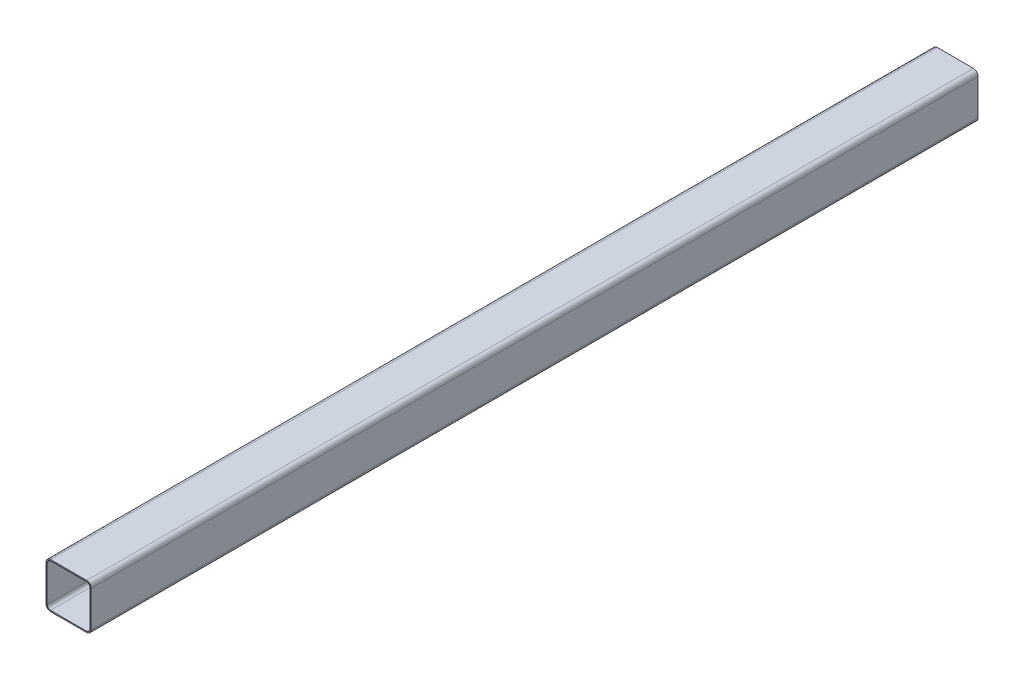
SolidWorks part; units mm, degrees
ref_plane "Front Plane" through (0, 0, 0) normal (0, 0, 1) x (1, 0, 0)
ref_plane "Top Plane" through (0, 0, 0) normal (0, 1, 0) x (1, 0, 0)
ref_plane "Right Plane" through (0, 0, 0) normal (1, 0, 0) x (0, 0, -1)
other "Configuration Table"
sketch "Sketch1" plane through (0, 0, 0) normal (0, 0, 1) x (1, 0, 0)
  line L0 (-95, 80) -> (-95, -80)
  line L1 (-80, 100) -> (80, 100)
  line L2 (-100, 80) -> (-100, -80)
  line L3 (-80, -100) -> (80, -100)
  line L4 (100, 80) -> (100, -80)
  line L5 (-100, 100) -> (100, -100) construction
  line L6 (-100, -100) -> (100, 100) construction
  line L7 (-80, -95) -> (80, -95)
  line L8 (95, 80) -> (95, -80)
  line L9 (-80, 95) -> (80, 95)
  arc A0 (-100, -80) -> (-80, -100) centre (-80, -80) ccw
  arc A1 (80, -100) -> (100, -80) centre (80, -80) ccw
  arc A2 (80, 100) -> (100, 80) centre (80, 80) cw
  arc A3 (-80, 100) -> (-100, 80) centre (-80, 80) ccw
  arc A4 (-95, -80) -> (-80, -95) centre (-80, -80) ccw
  arc A5 (80, -95) -> (95, -80) centre (80, -80) ccw
  arc A6 (80, 95) -> (95, 80) centre (80, 80) cw
  arc A7 (-80, 95) -> (-95, 80) centre (-80, 80) ccw
  point P0 (0, 0)
  dimension "D3" = 20
  dimension "D1" = 200
  dimension "D2" = 200
  dimension "D4" = 5
extrude "Boss-Extrude1" add sketch "Sketch1" along normal blind 3930
